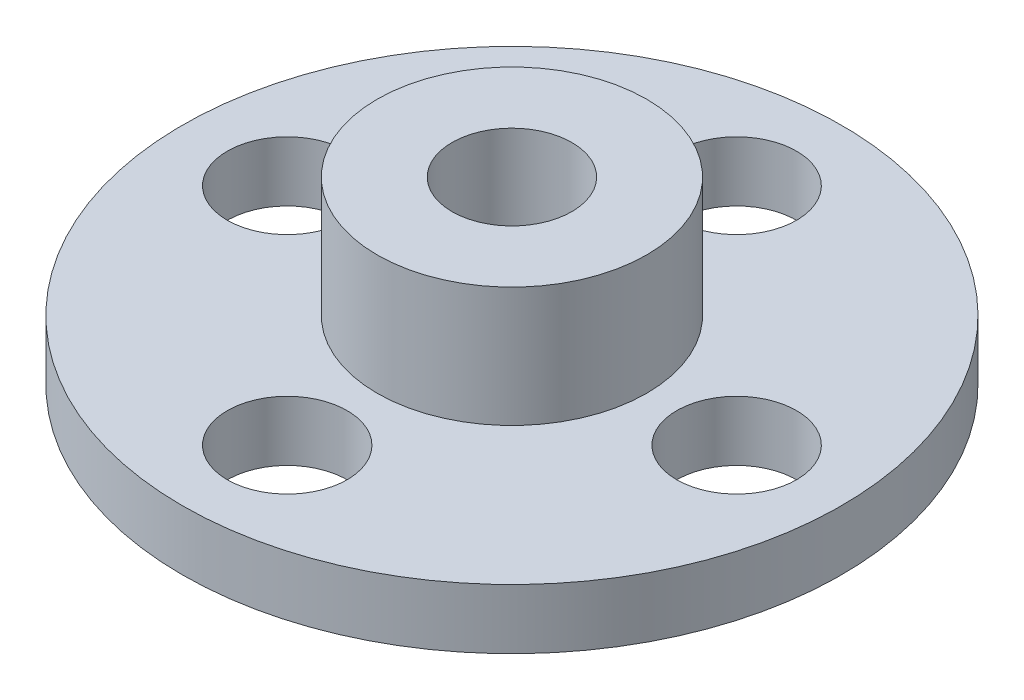
SolidWorks part; units mm, degrees
ref_plane "前视基准面" through (0, 0, 0) normal (0, 0, 1) x (1, 0, 0)
ref_plane "上视基准面" through (0, 0, 0) normal (0, 1, 0) x (1, 0, 0)
ref_plane "右视基准面" through (0, 0, 0) normal (1, 0, 0) x (0, 0, -1)
sketch "草图1" plane through (0, 0, 0) normal (0, 1, 0) x (1, 0, 0)
  circle A0 centre (0, 0) radius 11
  circle A1 centre (0, 0) radius 7.5 construction
  circle A2 centre (0, 7.5) radius 2
  circle A3 centre (7.5, 0) radius 2
  circle A4 centre (0, -7.5) radius 2
  circle A5 centre (-7.5, 0) radius 2
  point P15 (0, 0)
  dimension "D1" = 22
  dimension "D2" = 15
  dimension "D3" = 4
  dimension "D4" = 4
extrude "凸台-拉伸1" add sketch "草图1" along normal blind 2
sketch "草图2" plane through (0, 2, 0) normal (0, 1, 0) x (1, 0, 0)
  circle A0 centre (0, 0) radius 4.5
  dimension "D1" = 9
extrude "凸台-拉伸2" add sketch "草图2" along normal blind 4
sketch "草图3" plane through (0, 6, 0) normal (0, 1, 0) x (1, 0, 0)
  circle A0 centre (0, 0) radius 2
  dimension "D1" = 4
extrude "切除-拉伸1" cut sketch "草图3" against normal through all both and the other way through all
